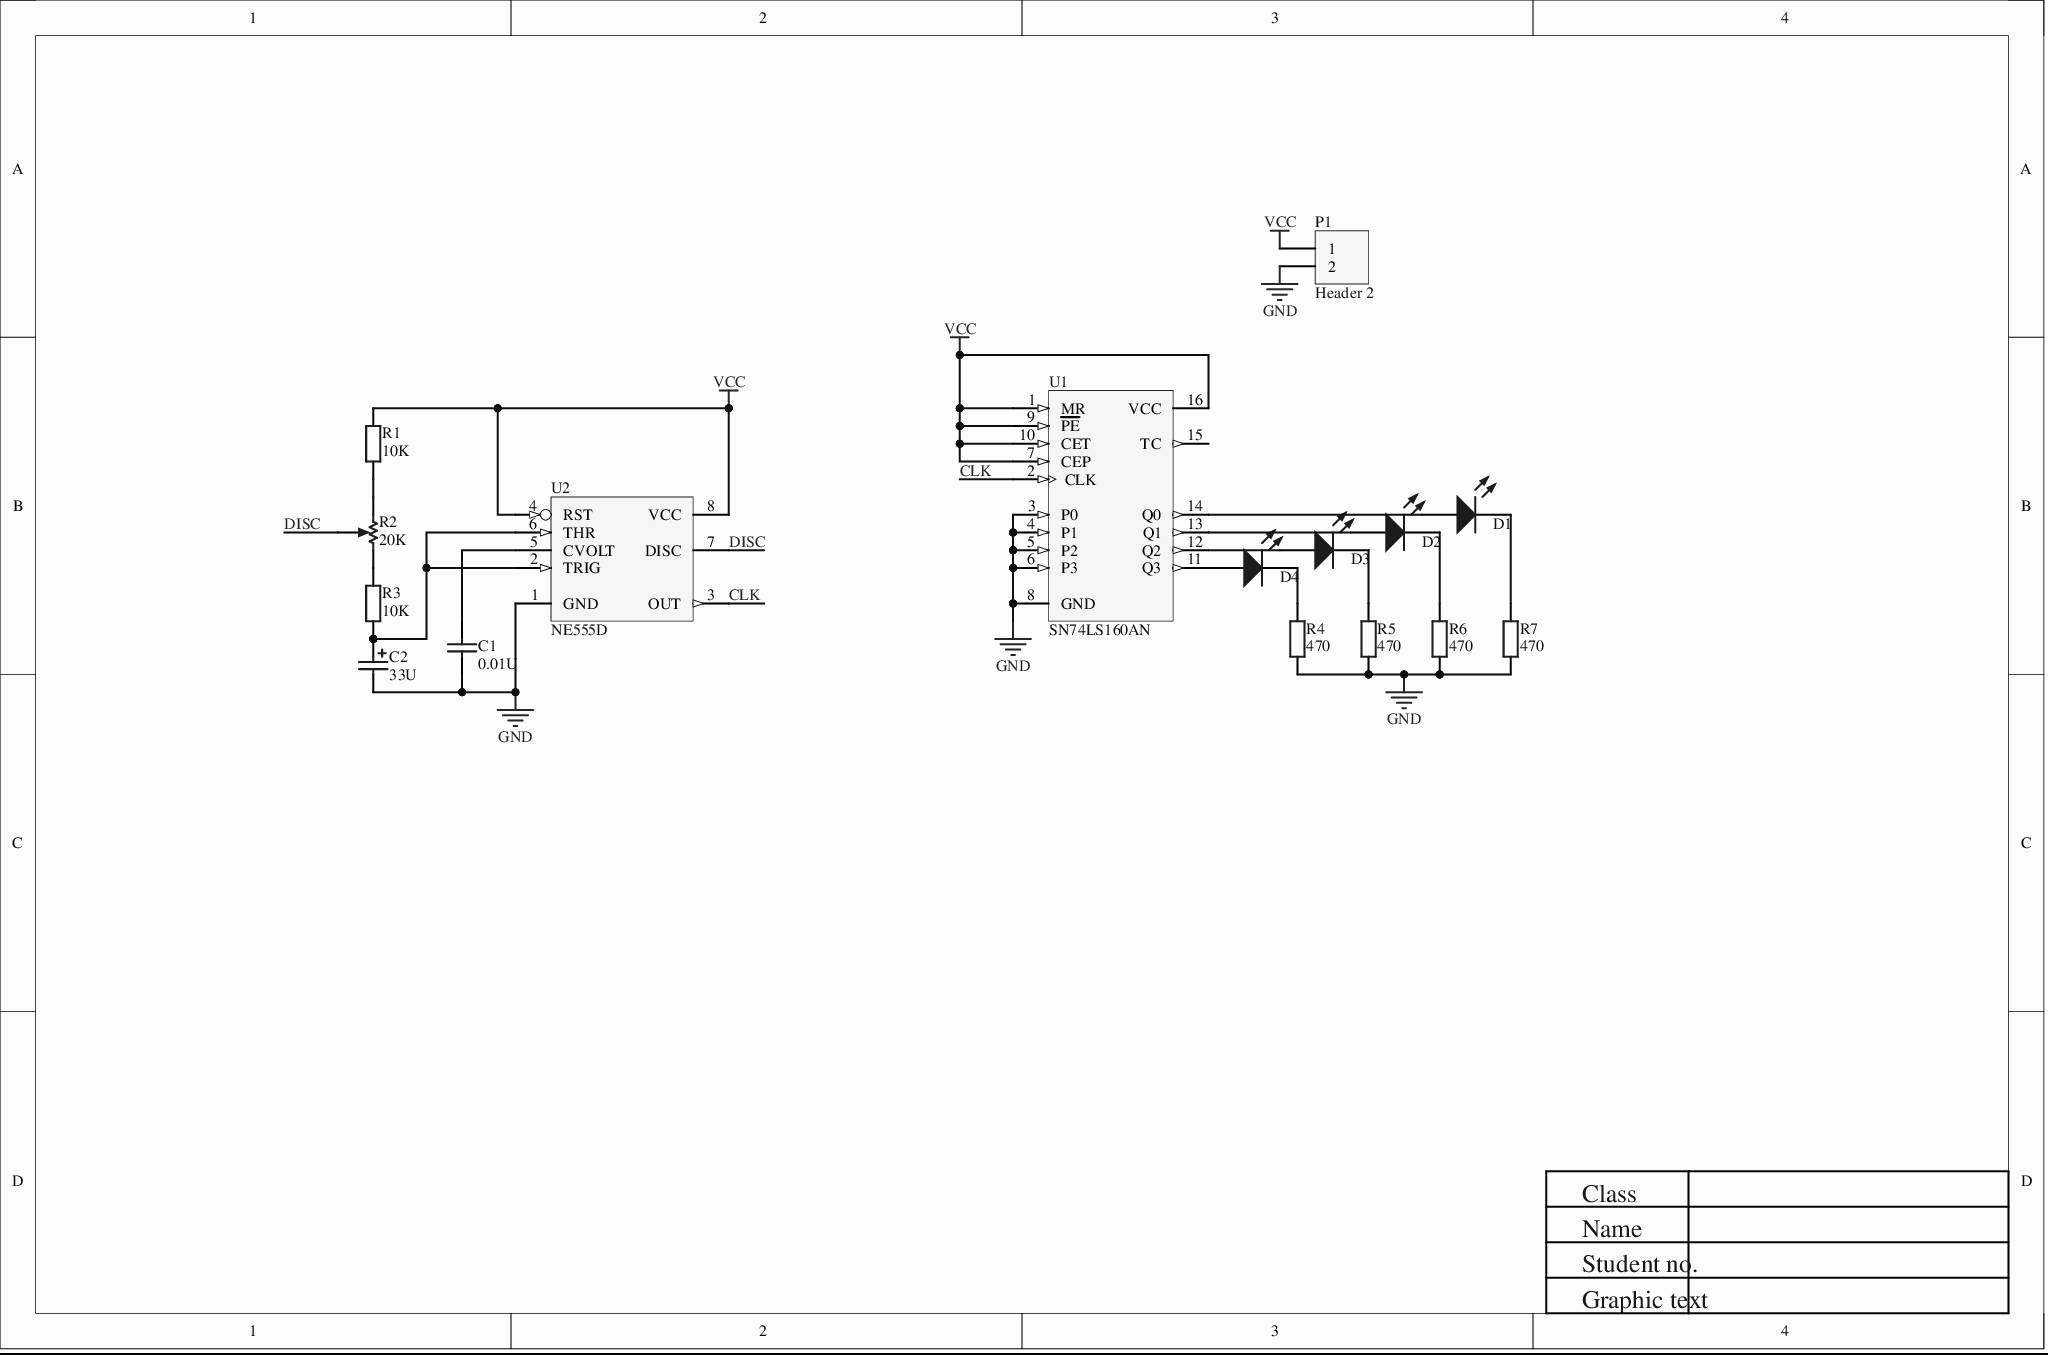
[diagram p0: MISC82778.SchDoc]
# Altium project MISC82778-8.PrjPcb
1 sheet, 16 parts. Net scope: global (net labels, ports and power ports of the same name join across sheets).
Board file: MISC82778.PcbDoc

## Sheet MISC82778.SchDoc
size A4

### Parts
C1  0.01U  [RAD-0.3]
C2  33U  [POLAR0.8]
D1  LED  [LED 5MM-W]  (value not drawn)
D2  LED  [LED 5MM-W]  (value not drawn)
D3  LED  [LED 5MM-W]  (value not drawn)
D4  LED  [LED 5MM-W]  (value not drawn)
P1  Header 2  [HDR1X2]
R1  10K  [RS 1/4W]
R2  20K  [VR5]
R3  10K  [RS 1/4W]
R4  470  [RS 1/4W]
R5  470  [RS 1/4W]
R6  470  [RS 1/4W]
R7  470  [RS 1/4W]
U1  SN74LS160AN  [648-08]
U2  NE555D  [DIP8]

### Nets
GND: C1.1 C2.2 P1.2 R4.1 R5.1 R6.1 R7.1 U1.3(P0) U1.4(P1) U1.5(P2) U1.6(P3) U1.8(GND) U2.1(GND)
VCC: P1.1 R1.2 U1.1(MR) U1.7(CEP) U1.9(~{PE}) U1.10(CET) U1.16(VCC) U2.4(RST) U2.8(VCC)
CLK: U1.2(CLK) U2.3(OUT)
DISC: R2.3(TAP) U2.7(DISC)
NetC1_2: C1.2 U2.5(CVOLT)
NetC2_1: C2.1 R3.1 U2.2(TRIG) U2.6(THR)
NetD1_1: D1.1(A) U1.14(Q0)
NetD1_2: D1.2(K) R7.2
NetD2_1: D2.1(A) U1.13(Q1)
NetD2_2: D2.2(K) R6.2
NetD3_1: D3.1(A) U1.12(Q2)
NetD3_2: D3.2(K) R5.2
NetD4_1: D4.1(A) U1.11(Q3)
NetD4_2: D4.2(K) R4.2
NetR1_1: R1.1 R2.1(TOP)
NetR2_2: R2.2(BOT) R3.2

Not connected (* = marked no-connect by the designer): U1 15(TC)

### Notes on the sheet
- Class
- Name
- Student no.
- Graphic text

### Library data of the parts
C1 = Cap: Capacitor; Value: 100pF; Published: 8-Jun-2000; LatestRevisionDate: 17-Jul-2002; LatestRevisionNote: Re-released for DXP Platform.; PackageReference: RAD-0.3; PackageDescription: Radial Cap, Thru-Hole; 2 Leads; 0.3 in Pin Spacing; Publisher: Altium Limited
C2 = Cap Pol2: Polarized Capacitor (Axial); Value: 100pF; Published: 8-Jun-2000; LatestRevisionDate: 17-Jul-2002; LatestRevisionNote: Re-released for DXP Platform.; PackageReference: POLAR0.8; PackageDescription: Polarized Capacitor; 2 Leads; Publisher: Altium Limited
D1-D4 = LED: Light-emitting diode
P1 = Header 2: Header, 2-Pin; LatestRevisionDate: 17-Jul-2002; LatestRevisionNote: Re-released for DXP Platform.; Publisher: Altium Limited
R1 R3-R7 = R-S: Color-band resistor; BOM名称: Color-band resistor
R2 = RPot: Potentiometer; Sim Note: Enter the Resistance value and the set point into parameter fields.; Set Position: 0.5; Value: 1K; Published: 8-Jun-2000; LatestRevisionDate: 17-Jul-2002; LatestRevisionNote: Re-released for DXP Platform.; PackageReference: VR5; PackageDescription: Variable Resistor, Thru-Hole; 3 Leads; Publisher: Altium Limited
U1 = SN74LS160AN: BCD Decade Counter; Package Information: Latest Revision: Apr-2000; Code - JEDEC: MS-001-BB; Published: 15-Apr-2002; Datasheet: Latest Revision: 18-Oct-1996; Package Reference: 648-08; Publisher: Altium Limited
U2 = NE555D: General-Purpose Single Bipolar Timer; Package Information: Latest Revision: Jul-1998; Code - JEDEC: MS-012-AA; Code - IPC: SO8; Published: 24-Aug-2001; Revision: 17-Jul-2002: Re-released for DXP Platform.; Datasheet: Latest Revision: Jul-1998; Package Reference: SO8; Publisher: Altium Limited